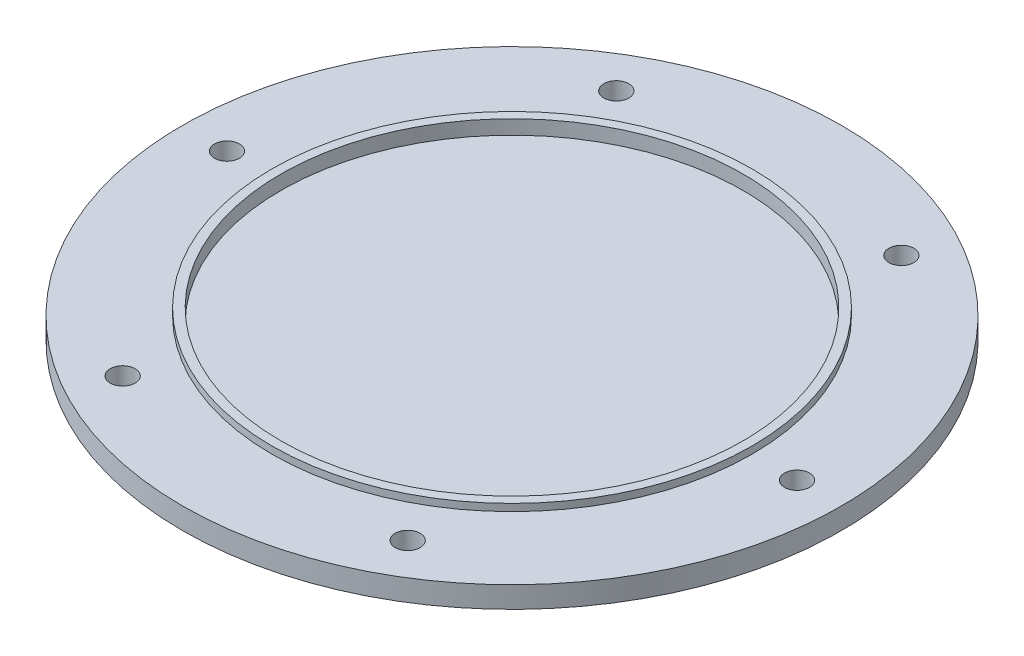
from build123d import *

# Parameters (mm, degrees)
SKETCH1_R           = 185
BOSS_EXTRUDE1_DEPTH = 12
SKETCH2_R           = 129.75
CUT_EXTRUDE1_DEPTH  = 4
BOSS_EXTRUDE2_START = 4
SKETCH3_R           = 134.75
SKETCH3_R_2         = 129.75
BOSS_EXTRUDE2_DEPTH = 4
SKETCH5_R           = 7
CUT_EXTRUDE3_DEPTH  = 262.90456277
CIRPATTERN2_COUNT   = 6


with BuildPart() as part:
    # Sketch1 → Boss-Extrude1 (new body)
    with BuildSketch(Plane(origin=(0, 0, 0), x_dir=(1, 0, 0), z_dir=(0, 1, 0))):
        with Locations(Location((0, 0, 0), (0, 0, 270))):
            Circle(SKETCH1_R)
    extrude(amount=BOSS_EXTRUDE1_DEPTH)

    # Sketch2 → Cut-Extrude1 (cut)
    with BuildSketch(Plane(origin=(0, 12, 0), x_dir=(1, 0, 0), z_dir=(0, 1, 0))):
        with Locations(Location((0, 0, 0), (0, 0, 270))):
            Circle(SKETCH2_R)
    extrude(amount=-CUT_EXTRUDE1_DEPTH, mode=Mode.SUBTRACT)

    # Sketch3 → Boss-Extrude2 (add)
    with BuildSketch(Plane(origin=(0, 12, 0), x_dir=(1, 0, 0), z_dir=(0, 1, 0)).offset(BOSS_EXTRUDE2_START)):
        with Locations(Location((0, 0, 0), (0, 0, 270))):
            Circle(SKETCH3_R)
        with Locations(Location((0, 0, 0), (0, 0, 270))):
            Circle(SKETCH3_R_2, mode=Mode.SUBTRACT)
    extrude(amount=-BOSS_EXTRUDE2_DEPTH)

    # Sketch5 → Cut-Extrude3 (cut, through all)
    with BuildSketch(Plane(origin=(0, 12, 0), x_dir=(1, 0, 0), z_dir=(0, 1, 0))):
        with Locations(Location((160, 0, 0), (0, 0, 270))):
            Circle(SKETCH5_R)
    cut_extrude3 = extrude(amount=-CUT_EXTRUDE3_DEPTH, mode=Mode.SUBTRACT)

    # CirPattern2: Cut-Extrude3 ×6 about axis
    cirpattern2_axis = Axis((0, 0, 0), (0, 1, 0))
    for i in range(1, CIRPATTERN2_COUNT):
        add(cut_extrude3.rotate(cirpattern2_axis, i * 360 / CIRPATTERN2_COUNT), mode=Mode.SUBTRACT)


solid = part.part
